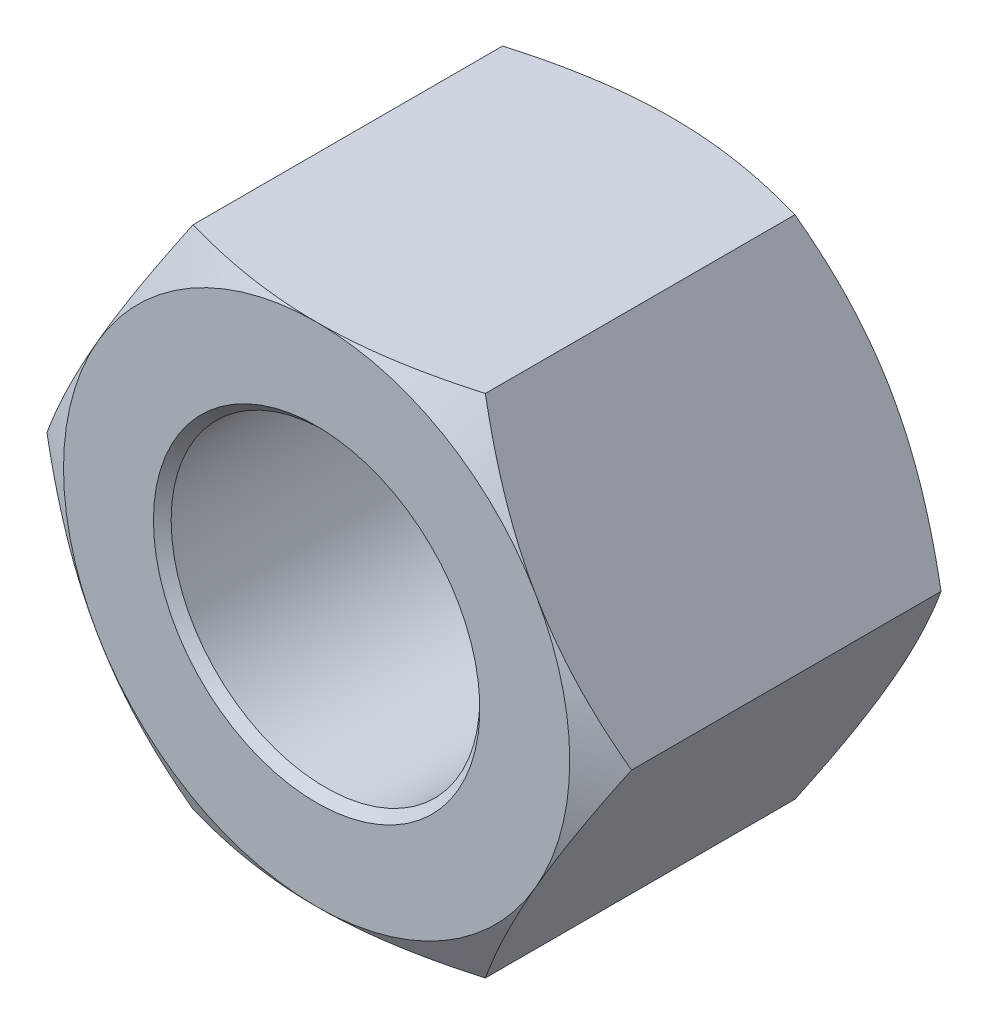
from build123d import *

# Parameters (mm, degrees)
SKETCH1_R          = 6.9175
BOSS_EXTRUDE_DEPTH = 15.9
SKETCH2_OUTSIDE_W  = 120.762
SKETCH2_OUTSIDE_H  = 117.252
SKETCH2_OUTSIDE_R  = 11.34493279
CUT_EXTRUDE1_DEPTH = 24.518662802
CUT_EXTRUDE1_DRAFT = -60
SKETCH3_OUTSIDE_W  = 120.762
SKETCH3_OUTSIDE_H  = 117.252
SKETCH3_OUTSIDE_R  = 11.34493279
CUT_EXTRUDE2_DEPTH = 24.518662802
CUT_EXTRUDE2_DRAFT = -60
CHAMFER1_SIZE      = 0.3975


with BuildPart() as part:
    # Sketch1 → Boss-Extrude (new body)
    with BuildSketch(Plane.XY):
        Polygon((6.55, 11.34493279), (-6.55, 11.34493279), (-13.1, 0), (-6.55, -11.34493279), (6.55, -11.34493279), (13.1, 0), align=None)
        Circle(SKETCH1_R, mode=Mode.SUBTRACT)
    extrude(amount=BOSS_EXTRUDE_DEPTH)


with BuildPart() as cut_extrude1_tool:
    # Sketch2 outside → Cut-Extrude1 (with draft: the straight prism first)
    with BuildSketch(Plane(origin=(0, 0, 0), x_dir=(-1, 0, 0), z_dir=(0, 0, -1))):
        Rectangle(SKETCH2_OUTSIDE_W, SKETCH2_OUTSIDE_H)
        Circle(SKETCH2_OUTSIDE_R, mode=Mode.SUBTRACT)
    extrude(amount=-CUT_EXTRUDE1_DEPTH)
    # Cut-Extrude1: the draft: its side faces are tilted about the plane it starts from
    cut_extrude1_sides = [cut_extrude1_tool.faces().sort_by_distance(p)[0] for p in [
        (0, -58.626, 12.259331401),
        (-60.381, 0, 12.259331401),
        (0, 58.626, 12.259331401),
        (60.381, 0, 12.259331401),
        (11.34493279, 0, 12.259331401),
    ]]
    draft(cut_extrude1_sides, Plane(origin=(0, 0, 0), x_dir=(-1, 0, 0), z_dir=(0, 0, -1)), CUT_EXTRUDE1_DRAFT)


with BuildPart() as part_1:
    add(part.part)

    # Cut-Extrude1: cut by cut_extrude1_tool
    add(cut_extrude1_tool.part, mode=Mode.SUBTRACT)


with BuildPart() as cut_extrude2_tool:
    # Sketch3 outside → Cut-Extrude2 (with draft: the straight prism first)
    with BuildSketch(Plane.XY.offset(15.9)):
        Rectangle(SKETCH3_OUTSIDE_W, SKETCH3_OUTSIDE_H)
        Circle(SKETCH3_OUTSIDE_R, mode=Mode.SUBTRACT)
    extrude(amount=-CUT_EXTRUDE2_DEPTH)
    # Cut-Extrude2: the draft: its side faces are tilted about the plane it starts from
    cut_extrude2_sides = [cut_extrude2_tool.faces().sort_by_distance(p)[0] for p in [
        (0, -58.626, 3.640668599),
        (60.381, 0, 3.640668599),
        (0, 58.626, 3.640668599),
        (-60.381, 0, 3.640668599),
        (-11.34493279, 0, 3.640668599),
    ]]
    draft(cut_extrude2_sides, Plane.XY.offset(15.9), CUT_EXTRUDE2_DRAFT)


with BuildPart() as part_2:
    add(part_1.part)

    # Cut-Extrude2: cut by cut_extrude2_tool
    add(cut_extrude2_tool.part, mode=Mode.SUBTRACT)

    # Chamfer1
    chamfer1_edges = [part_2.edges().sort_by_distance(p)[0] for p in [
        (-6.9175, 0, 0),
        (-6.9175, 0, 15.9),
    ]]
    chamfer(chamfer1_edges, length=CHAMFER1_SIZE)


solid = part_2.part
